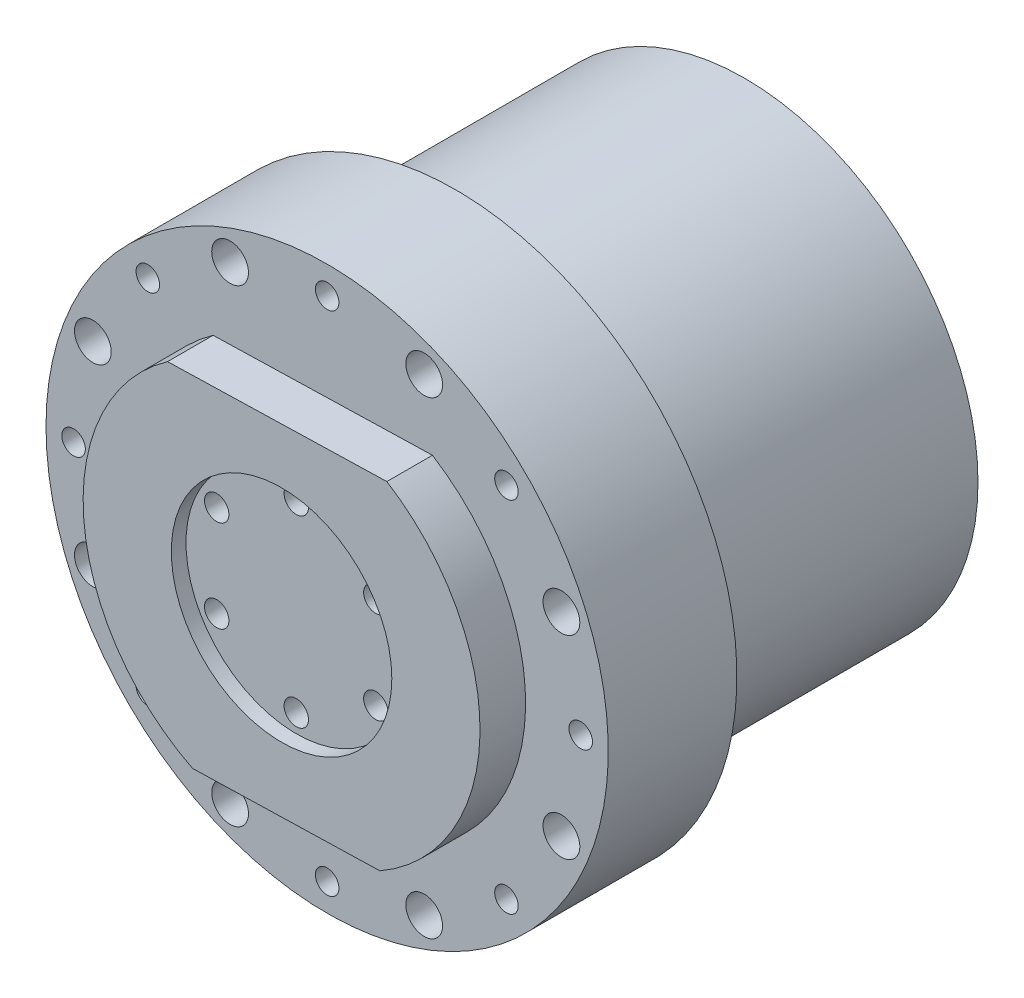
from build123d import *

# Parameters (mm, degrees)
SKETCH1_R           = 1.66
BOSS_EXTRUDE1_DEPTH = 6.2
SKETCH2_R           = 38.25
SKETCH2_R_2         = 1.6
SKETCH2_R_3         = 2.5
BOSS_EXTRUDE2_DEPTH = 17.5
SKETCH3_R           = 31.75
BOSS_EXTRUDE3_DEPTH = 39.3
SKETCH4_R           = 15
CUT_EXTRUDE1_DEPTH  = 2


with BuildPart() as part:
    # Sketch1 → Boss-Extrude1 (new body)
    with BuildSketch(Plane.XY):
        with BuildLine():
            Line((-15.516105129, 22.096390692), (14.325275898, 22.886381768))
            ThreePointArc((14.325275898, 22.886381768), (26.994312242, -0.554171996), (13.373923279, -23.455024539))
            Line((13.373923279, -23.455024539), (-12.114210645, -24.129772076))
            ThreePointArc((-12.114210645, -24.129772076), (-26.927181778, -1.981636062), (-15.516105129, 22.096390692))
        make_face()
        with Locations(Location((0, 12.5, 0), (0, 0, 180))):
            Circle(SKETCH1_R, mode=Mode.SUBTRACT)
        with Locations(Location((10.825317547, 6.25, 0), (0, 0, 180))):
            Circle(SKETCH1_R, mode=Mode.SUBTRACT)
        with Locations(Location((0, -12.5, 0), (0, 0, 180))):
            Circle(SKETCH1_R, mode=Mode.SUBTRACT)
        with Locations(Location((10.825317547, -6.25, 0), (0, 0, 180))):
            Circle(SKETCH1_R, mode=Mode.SUBTRACT)
        with Locations(Location((-10.825317547, -6.25, 0), (0, 0, 180))):
            Circle(SKETCH1_R, mode=Mode.SUBTRACT)
        with Locations(Location((-10.825317547, 6.25, 0), (0, 0, 180))):
            Circle(SKETCH1_R, mode=Mode.SUBTRACT)
    extrude(amount=BOSS_EXTRUDE1_DEPTH)

    # Sketch2 → Boss-Extrude2 (add)
    with BuildSketch(Plane(origin=(0, 0, 0), x_dir=(-1, 0, 0), z_dir=(0, 0, -1))):
        Circle(SKETCH2_R)
        with Locations((0, 34.5)):
            Circle(SKETCH2_R_2, mode=Mode.SUBTRACT)
        with Locations(Location((24.395183951, 24.395183951, 0), (0, 0, 180))):
            Circle(SKETCH2_R_2, mode=Mode.SUBTRACT)
        with Locations((34.5, 0)):
            Circle(SKETCH2_R_2, mode=Mode.SUBTRACT)
        with Locations(Location((24.395183951, -24.395183951, 0), (0, 0, 180))):
            Circle(SKETCH2_R_2, mode=Mode.SUBTRACT)
        with Locations(Location((0, -34.5, 0), (0, 0, 180))):
            Circle(SKETCH2_R_2, mode=Mode.SUBTRACT)
        with Locations((-24.395183951, -24.395183951)):
            Circle(SKETCH2_R_2, mode=Mode.SUBTRACT)
        with Locations(Location((-34.5, 0, 0), (0, 0, 180))):
            Circle(SKETCH2_R_2, mode=Mode.SUBTRACT)
        with Locations((-24.395183951, 24.395183951)):
            Circle(SKETCH2_R_2, mode=Mode.SUBTRACT)
        with Locations((13.202578417, 31.873843872)):
            Circle(SKETCH2_R_3, mode=Mode.SUBTRACT)
        with Locations(Location((31.873843872, 13.202578417, 0), (0, 0, 180))):
            Circle(SKETCH2_R_3, mode=Mode.SUBTRACT)
        with Locations((31.873843872, -13.202578417)):
            Circle(SKETCH2_R_3, mode=Mode.SUBTRACT)
        with Locations(Location((13.202578417, -31.873843872, 0), (0, 0, 180))):
            Circle(SKETCH2_R_3, mode=Mode.SUBTRACT)
        with Locations((-31.873843872, -13.202578417)):
            Circle(SKETCH2_R_3, mode=Mode.SUBTRACT)
        with Locations(Location((-31.873843872, 13.202578417, 0), (0, 0, 180))):
            Circle(SKETCH2_R_3, mode=Mode.SUBTRACT)
        with Locations((-13.202578417, 31.873843872)):
            Circle(SKETCH2_R_3, mode=Mode.SUBTRACT)
        with Locations(Location((-13.202578417, -31.873843872, 0), (0, 0, 180))):
            Circle(SKETCH2_R_3, mode=Mode.SUBTRACT)
    extrude(amount=BOSS_EXTRUDE2_DEPTH)

    # Sketch3 → Boss-Extrude3 (add)
    with BuildSketch(Plane(origin=(0, 0, -17.5), x_dir=(-1, 0, 0), z_dir=(0, 0, -1))):
        Circle(SKETCH3_R)
    extrude(amount=BOSS_EXTRUDE3_DEPTH)

    # Sketch4 → Cut-Extrude1 (cut)
    with BuildSketch(Plane.XY.offset(6.2)):
        Circle(SKETCH4_R)
    extrude(amount=-CUT_EXTRUDE1_DEPTH, mode=Mode.SUBTRACT)


solid = part.part
